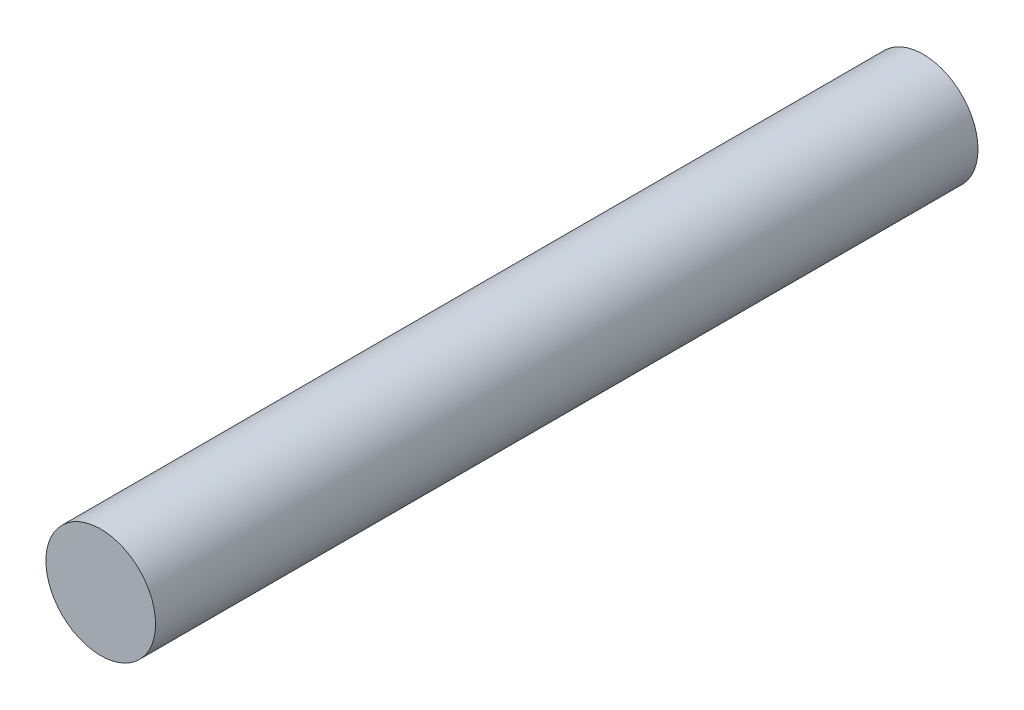
SolidWorks part; units mm, degrees
ref_plane "Front Plane" through (0, 0, 0) normal (0, 0, 1) x (1, 0, 0)
ref_plane "Top Plane" through (0, 0, 0) normal (0, 1, 0) x (1, 0, 0)
ref_plane "Right Plane" through (0, 0, 0) normal (1, 0, 0) x (0, 0, -1)
sketch "Sketch1" plane through (0, 0, 0) normal (0, 0, 1) x (1, 0, 0)
  circle A0 centre (0, 0) radius 10
  dimension "D1" = 20
extrude "Boss-Extrude1" add sketch "Sketch1" along normal blind 150
